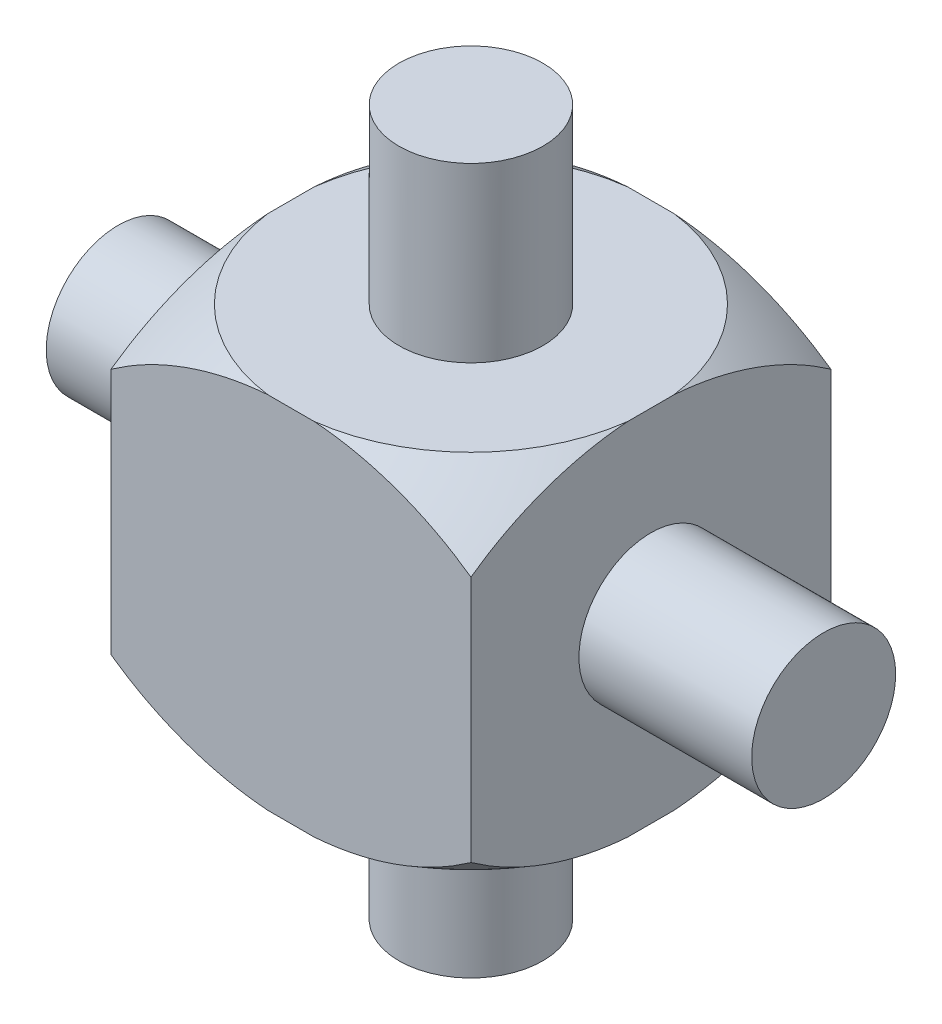
from build123d import *

# Parameters (mm, degrees)
EXTRUDE_1_DEPTH      = 12.5
EXTRUDE_1_DEPTH_BACK = 12.5
SKETCH_1_W           = 25
SKETCH_1_H           = 25
EXTRUDE_2_DEPTH      = 24.5
EXTRUDE_2_DEPTH_BACK = 24.5
SKETCH_4_R           = 5
EXTRUDE_3_DEPTH      = 24.5
EXTRUDE_3_DEPTH_BACK = 24.5
SKETCH_5_R           = 5


with BuildPart() as part:
    # 草图1 → 凸台-拉伸1 (new, two sides: drawn at the far end of the back side and taken through both)
    with BuildSketch(Plane(origin=(0, 0, 0), x_dir=(0, 0, -1), z_dir=(1, 0, 0)).offset(-EXTRUDE_1_DEPTH_BACK)):
        Rectangle(SKETCH_1_W, SKETCH_1_H)
    extrude(amount=EXTRUDE_1_DEPTH + EXTRUDE_1_DEPTH_BACK)

    # 草图2 → 切除-旋转1 (revolve, cut)
    with BuildSketch(Plane(origin=(0, 0, 0), x_dir=(0, 0, -1), z_dir=(1, 0, 0))):
        with BuildLine():
            Line((0, -25), (-25, -25))
            Line((-25, -25), (-25, 9.090909091))
            ThreePointArc((-25, 9.090909091), (-17.67766953, -8.586760439), (0, -15.909090909))
            Line((0, -15.909090909), (0, -25))
        make_face()
    revolve(axis=Axis((0, -15.909090909, 0), (0, -1, 0)), mode=Mode.SUBTRACT)

    # 草图3 → 切除-旋转2 (revolve, cut)
    with BuildSketch(Plane(origin=(0, 0, 0), x_dir=(0, 0, -1), z_dir=(1, 0, 0))):
        with BuildLine():
            Line((0, 25), (25, 25))
            Line((25, 25), (25, -9.090909091))
            ThreePointArc((25, -9.090909091), (17.67766953, 8.586760439), (0, 15.909090909))
            Line((0, 15.909090909), (0, 25))
        make_face()
    revolve(axis=Axis((0, 15.909090909, 0), (0, 1, 0)), mode=Mode.SUBTRACT)

    # 草图4 → 凸台-拉伸2 (add, two sides: drawn at the far end of the back side and taken through both)
    with BuildSketch(Plane(origin=(0, 0, 0), x_dir=(1, 0, 0), z_dir=(0, 1, 0)).offset(-EXTRUDE_2_DEPTH_BACK)):
        with Locations(Location((0, 0, 0), (0, 0, 270))):
            Circle(SKETCH_4_R)
    extrude(amount=EXTRUDE_2_DEPTH + EXTRUDE_2_DEPTH_BACK)

    # 草图5 → 凸台-拉伸3 (add, two sides: drawn at the far end of the back side and taken through both)
    with BuildSketch(Plane(origin=(0, 0, 0), x_dir=(0, 0, -1), z_dir=(1, 0, 0)).offset(-EXTRUDE_3_DEPTH_BACK)):
        Circle(SKETCH_5_R)
    extrude(amount=EXTRUDE_3_DEPTH + EXTRUDE_3_DEPTH_BACK)


solid = part.part
